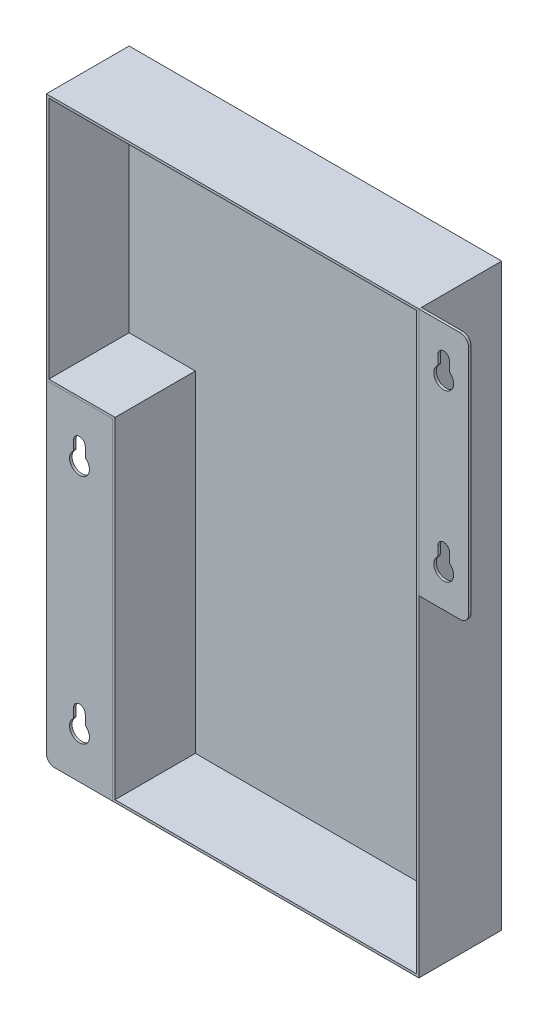
from build123d import *

# Parameters (mm, degrees)
SKETCH_1_W          = 225
SKETCH_1_H          = 350
EXTRUDE_1_DEPTH     = 50
SKETCH_2_W          = 40
SKETCH_2_H          = 200
CUT_EXTRUDE_1_DEPTH = 214.965534608
SHELL_1_T           = -1.5
SKETCH_3_W          = 40
SKETCH_3_H          = 200
EXTRUDE_2_DEPTH     = 1.5
SKETCH_3_W_2        = 30
SKETCH_3_H_2        = 150
EXTRUDE_2_2_DEPTH   = 1.5
FILLET_1_R          = 5
FILLET_2_R          = 5
CUT_EXTRUDE_4_DEPTH = 232.152006264


with BuildPart() as part:
    # 草图1 → 凸台-拉伸1 (new body)
    with BuildSketch(Plane.XY):
        Rectangle(SKETCH_1_W, SKETCH_1_H)
    extrude(amount=EXTRUDE_1_DEPTH)

    # 草图2 → 切除-拉伸1 (cut, through all)
    with BuildSketch(Plane(origin=(0, 0, 0), x_dir=(-1, 0, 0), z_dir=(0, 0, -1))):
        with Locations((92.5, -75)):
            Rectangle(SKETCH_2_W, SKETCH_2_H)
    extrude(amount=-CUT_EXTRUDE_1_DEPTH, mode=Mode.SUBTRACT)

    # 抽壳1
    shell_1_openings = [part.faces().sort_by_distance(p)[0] for p in [
        (10.459363958, 8.480565371, 50),
    ]]
    offset(amount=SHELL_1_T, openings=shell_1_openings, kind=Kind.INTERSECTION)


with BuildPart() as body_2:
    # 草图3 → 凸台-拉伸2 (new body)
    with BuildSketch(Plane.XY.offset(50)):
        with Locations((-92.5, -75)):
            Rectangle(SKETCH_3_W, SKETCH_3_H)
    extrude(amount=-EXTRUDE_2_DEPTH)

    # 圆角2
    fillet_2_edges = [body_2.edges().sort_by_distance(p)[0] for p in [
        (-112.5, -175, 49.25),
    ]]
    fillet(fillet_2_edges, radius=FILLET_2_R)


with BuildPart() as body_3:
    # 草图3 → Extrude 2 2 (new body)
    with BuildSketch(Plane.XY.offset(50)):
        with Locations((127.5, 100)):
            Rectangle(SKETCH_3_W_2, SKETCH_3_H_2)
    extrude(amount=-EXTRUDE_2_2_DEPTH)

    # 圆角1
    fillet_1_edges = [body_3.edges().sort_by_distance(p)[0] for p in [
        (142.5, 175, 49.25),
        (142.5, 25, 49.25),
    ]]
    fillet(fillet_1_edges, radius=FILLET_1_R)


with BuildPart() as cut_extrude_4_tool:
    # 草图4 → 切除-拉伸4 (new, through all)
    with BuildSketch(Plane(origin=(0, 0, 0), x_dir=(-1, 0, 0), z_dir=(0, 0, -1))):
        with BuildLine():
            Line((96, 2.292420126), (96, -2.707579874))
            ThreePointArc((96, -2.707579874), (96.162882693, -3.498149289), (96.625, -4.159948629))
            ThreePointArc((96.625, -4.159948629), (92.5, -14.517054893), (88.375, -4.159948629))
            ThreePointArc((88.375, -4.159948629), (88.837117307, -3.498149289), (89, -2.707579874))
            Line((89, -2.707579874), (89, 2.292420126))
            ThreePointArc((89, 2.292420126), (92.5, 5.792420126), (96, 2.292420126))
        make_face()
        with BuildLine():
            Line((96, -137.707579874), (96, -142.707579874))
            ThreePointArc((96, -142.707579874), (96.162882693, -143.498149289), (96.625, -144.159948629))
            ThreePointArc((96.625, -144.159948629), (92.5, -154.517054893), (88.375, -144.159948629))
            ThreePointArc((88.375, -144.159948629), (88.837117307, -143.498149289), (89, -142.707579874))
            Line((89, -142.707579874), (89, -137.707579874))
            ThreePointArc((89, -137.707579874), (92.5, -134.207579874), (96, -137.707579874))
        make_face()
        with BuildLine():
            Line((-124, 157), (-124, 152))
            ThreePointArc((-124, 152), (-123.837117307, 151.209430585), (-123.375, 150.547631245))
            ThreePointArc((-123.375, 150.547631245), (-127.5, 140.190524981), (-131.625, 150.547631245))
            ThreePointArc((-131.625, 150.547631245), (-131.162882693, 151.209430585), (-131, 152))
            Line((-131, 152), (-131, 157))
            ThreePointArc((-131, 157), (-127.5, 160.5), (-124, 157))
        make_face()
        with BuildLine():
            Line((-124, 57), (-124, 52))
            ThreePointArc((-124, 52), (-123.837117307, 51.209430585), (-123.375, 50.547631245))
            ThreePointArc((-123.375, 50.547631245), (-127.5, 40.190524981), (-131.625, 50.547631245))
            ThreePointArc((-131.625, 50.547631245), (-131.162882693, 51.209430585), (-131, 52))
            Line((-131, 52), (-131, 57))
            ThreePointArc((-131, 57), (-127.5, 60.5), (-124, 57))
        make_face()
    extrude(amount=-CUT_EXTRUDE_4_DEPTH)


with BuildPart() as body_2_1:
    add(body_2.part)

    # 切除-拉伸4: cut by cut_extrude_4_tool
    add(cut_extrude_4_tool.part, mode=Mode.SUBTRACT)


with BuildPart() as body_3_1:
    add(body_3.part)

    # 切除-拉伸4: cut by cut_extrude_4_tool
    add(cut_extrude_4_tool.part, mode=Mode.SUBTRACT)


solid = Compound([part.part, body_2_1.part, body_3_1.part])
